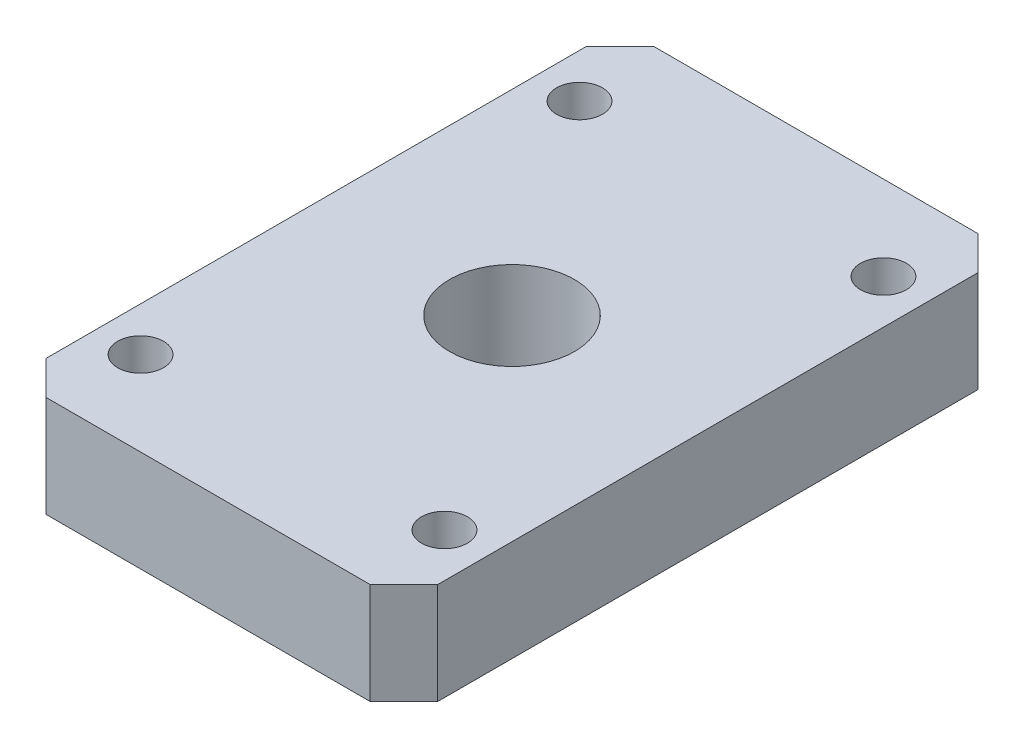
from build123d import *

# Parameters (mm, degrees)
SKETCH_1_W             = 58
SKETCH_1_H             = 90
EXTRUDE_1_DEPTH        = 7.5
HOLE_WIZARD_M8_1_D     = 6.8
HOLE_WIZARD_M8_1_DEPTH = 19.75
HOLE_WIZARD_M8_1_TIP   = 2.042926105
M20X1_5_1_D            = 18.5
M20X1_5_1_DEPTH        = 44.5
M20X1_5_1_TIP          = 5.557960726
CHAMFER_1_SIZE         = 5


with BuildPart() as part:
    # 草图1 → 凸台-拉伸1 (new, symmetric)
    with BuildSketch(Plane(origin=(0, 0, 0), x_dir=(1, 0, 0), z_dir=(0, 1, 0))):
        Rectangle(SKETCH_1_W, SKETCH_1_H)
    extrude(amount=EXTRUDE_1_DEPTH, both=True)

    # M8 螺纹孔1
    with Locations(Plane.XZ.offset(7.5)):
        with Locations((-22.5, -32.5), (22.5, -32.5), (22.5, 32.5), (-22.5, 32.5)):
            Hole(HOLE_WIZARD_M8_1_D / 2, depth=HOLE_WIZARD_M8_1_DEPTH)
            with Locations((0, 0, -(HOLE_WIZARD_M8_1_DEPTH + HOLE_WIZARD_M8_1_TIP / 2))):  # 118° drill point
                Cone(0, HOLE_WIZARD_M8_1_D / 2, HOLE_WIZARD_M8_1_TIP, mode=Mode.SUBTRACT)

    # M20x1.5 螺纹孔1
    with Locations(Plane(origin=(0, 7.5, 0), x_dir=(1, 0, 0), z_dir=(0, 1, 0))):
        with Locations((0, 0)):
            Hole(M20X1_5_1_D / 2, depth=M20X1_5_1_DEPTH)
            with Locations((0, 0, -(M20X1_5_1_DEPTH + M20X1_5_1_TIP / 2))):  # 118° drill point
                Cone(0, M20X1_5_1_D / 2, M20X1_5_1_TIP, mode=Mode.SUBTRACT)

    # 倒角1
    chamfer_1_edges = [part.edges().sort_by_distance(p)[0] for p in [
        (29, 0, 45),
        (-29, 0, 45),
        (-29, 0, -45),
        (29, 0, -45),
    ]]
    chamfer(chamfer_1_edges, length=CHAMFER_1_SIZE)


solid = part.part
